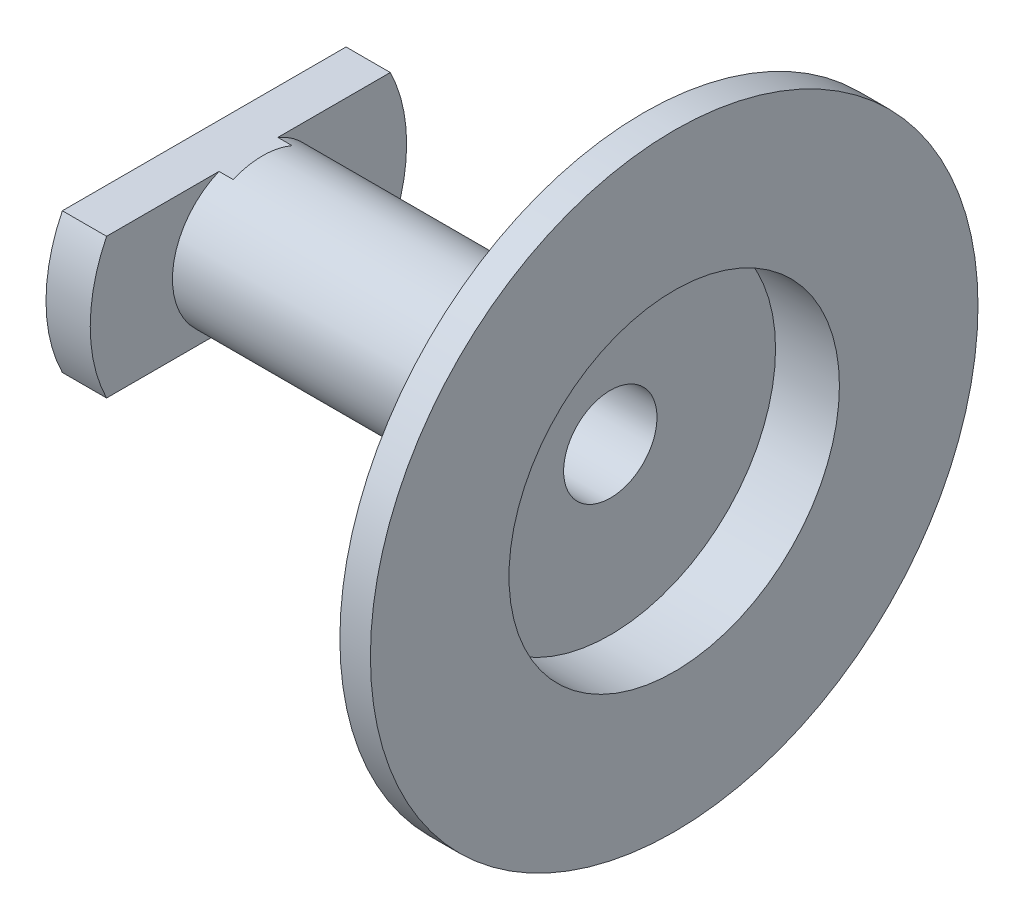
SolidWorks part; units mm, degrees
ref_plane "Front Plane" through (0, 0, 0) normal (0, 0, 1) x (1, 0, 0)
ref_plane "Top Plane" through (0, 0, 0) normal (0, 1, 0) x (1, 0, 0)
ref_plane "Right Plane" through (0, 0, 0) normal (1, 0, 0) x (0, 0, -1)
sketch "Sketch1" plane through (0, 0, 0) normal (0, 0, 1) x (1, 0, 0)
  line L0 (0, 0) -> (-27.1764, 0) construction
  line L1 (-74.1426, 26.0243) -> (-74.1426, 17.4546)
  line L2 (-74.1426, -33.4546) -> (-74.1426, 33.4546) construction
  line L3 (-74.1426, -17.4546) -> (-74.1426, 17.4546) construction
  line L4 (-74.1426, 17.4546) -> (-79.307, 17.4546)
  line L5 (-79.307, 17.4546) -> (-79.307, 6.5082)
  line L6 (-79.307, 6.5082) -> (-108, 6.5082)
  line L7 (-109.9542, 31.426) -> (-109.9542, -31.426) construction
  line L8 (-106.2675, 4) -> (-111.789, 4)
  line L11 (-104, 4) -> (-107, 4) construction
  line L12 (-106.2675, 4) -> (-77, 4)
  line L13 (-77, 20.4546) -> (-77, -20.4546) construction
  line L14 (-77, 4) -> (-77, 14.1537)
  line L15 (-77, 14.1537) -> (-71.5273, 14.1537)
  line L16 (-71.5273, 14.1537) -> (-71.5273, 26.0243)
  line L17 (-71.5273, 26.0243) -> (-74.1426, 26.0243)
  line L18 (-108, 6.5082) -> (-108, 13.5517)
  line L19 (-108, 24.55) -> (-108, -24.55) construction
  line L20 (-108, 13.5517) -> (-109.9542, 13.5517)
  line L23 (-109.9542, 13.5517) -> (-111.789, 13.5517)
  line L26 (-111.789, 13.5517) -> (-111.789, 4)
revolve "Revolve1" add sketch "Sketch1" angle 360 about L0
sketch "Sketch2" plane through (-111.789, 0, 0) normal (-1, 0, 0) x (0, 0, 1)
  line L1 (-44.6041, 21.5928) -> (37.9619, 21.5928)
  line L2 (-44.6041, 21.5928) -> (-44.6041, 6)
  line L3 (-44.6041, 6) -> (37.9619, 6)
  line L4 (37.9619, 21.5928) -> (37.9619, 6)
  line L5 (79.9962, -6) -> (-68.9709, -6)
  line L6 (79.9962, -6) -> (79.9962, -17.9581)
  line L7 (79.9962, -17.9581) -> (-68.9709, -17.9581)
  line L8 (-68.9709, -6) -> (-68.9709, -17.9581)
  circle A1 centre (0, 0) radius 4 construction
  dimension "D1" = 6
  dimension "D2" = 6
extrude "Cut-Extrude1" cut sketch "Sketch2" against normal blind 5 contours L4 L3 L2 L1
